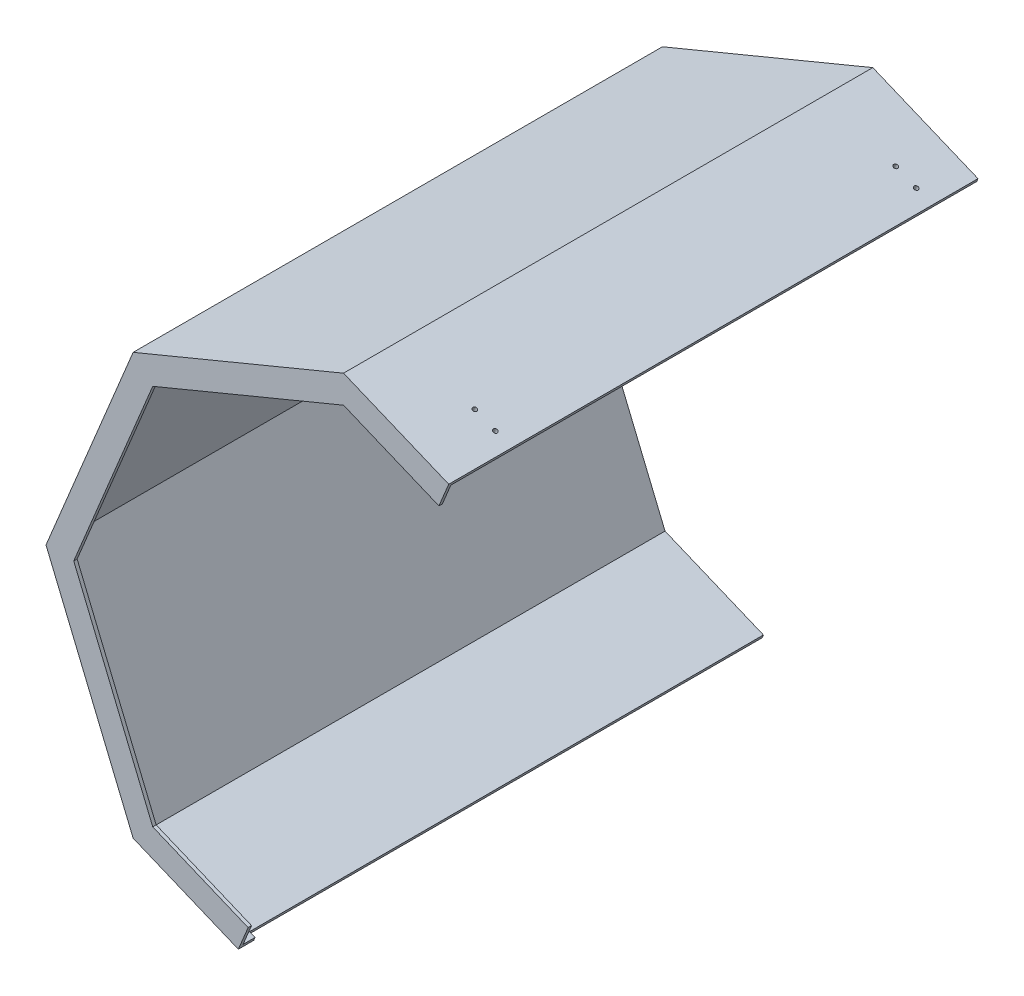
from build123d import *

# Parameters (mm, degrees)
BOSS_EXTRUDE1_DEPTH   = 310
SHELL1_T              = -2
CUT_EXTRUDE1_DEPTH    = 10
CUT_EXTRUDE2_DEPTH    = 397.026111511
SKETCH4_R             = 3
BOSS_EXTRUDE2_DEPTH   = 2
M3_TAPPED_HOLE1_D     = 2.5
M3_TAPPED_HOLE1_DEPTH = 4
CUT_EXTRUDE3_REACH    = 466.348
SKETCH7_W             = 3.5
SKETCH7_H             = 301


with BuildPart() as part:
    # Sketch1 → Boss-Extrude1 (new body)
    with BuildSketch(Plane.XY):
        Polygon((-174.265144247, 0), (-123.224065222, -123.224065222), (0, -174.265144247), (123.224065222, -123.224065222), (174.265144247, 0), (123.224065222, 123.224065222), (0, 174.265144247), (-123.224065222, 123.224065222), align=None)
    extrude(amount=BOSS_EXTRUDE1_DEPTH)

    # Shell1
    shell1_openings = [part.faces().sort_by_distance(p)[0] for p in [
        (0, 0, 0),
    ]]
    offset(amount=SHELL1_T, openings=shell1_openings, kind=Kind.INTERSECTION)

    # Sketch2 → Cut-Extrude1 (cut)
    with BuildSketch(Plane.XY.offset(310)):
        Polygon((111.743562251, 111.743562251), (0, 158.029261243), (-111.743562251, 111.743562251), (-158.029261243, 0), (-111.743562251, -111.743562251), (0, -158.029261243), (111.743562251, -111.743562251), (158.029261243, 0), align=None)
    extrude(amount=-CUT_EXTRUDE1_DEPTH, mode=Mode.SUBTRACT)

    # Sketch3 → Cut-Extrude2 (cut, through all)
    with BuildSketch(Plane.XY.offset(310)):
        Polygon((70.138181093, 169.328548035), (-63.801020235, -154.029288344), (130.028007017, -234.315900213), (263.967208344, 89.041936166), align=None)
    extrude(amount=-CUT_EXTRUDE2_DEPTH, mode=Mode.SUBTRACT)

    # Sketch4 → Boss-Extrude2 (add)
    with BuildSketch(Plane(origin=(60.846665746, 146.896845669, 0), x_dir=(0.9238795325112958, -0.38268343236506785, 0), z_dir=(-0.38268343236506785, -0.9238795325112958, 0))):
        with Locations((-23.217589358, 273.25)):
            Circle(SKETCH4_R)
        with Locations((-10.217589358, 273.25)):
            Circle(SKETCH4_R)
        with Locations((-10.217589358, 26.75)):
            Circle(SKETCH4_R)
        with Locations((-23.217589358, 26.75)):
            Circle(SKETCH4_R)
    extrude(amount=BOSS_EXTRUDE2_DEPTH)

    # M3 Tapped Hole1
    with Locations(Plane(origin=(61.612032611, 148.744604734, 0), x_dir=(0.9238795325112958, -0.38268343236506785, 0), z_dir=(0.38268343236506785, 0.9238795325112958, 0))):
        with Locations((-23.217589358, -26.75), (-10.217589358, -26.75), (-23.217589358, -273.25), (-10.217589358, -273.25)):
            Hole(M3_TAPPED_HOLE1_D / 2, depth=M3_TAPPED_HOLE1_DEPTH)

    # Sketch7 → Cut-Extrude3 (cut, up to next)
    with BuildSketch(Plane(origin=(-61.612032611, -148.744604734, 0), x_dir=(0.9238795325112957, -0.38268343236506797, 0), z_dir=(-0.38268343236506797, -0.9238795325112957, 0)), mode=Mode.PRIVATE) as cut_extrude3_sk1:
        with Locations((-1.75, 150.5)):
            Rectangle(SKETCH7_W, SKETCH7_H)
    cut_extrude3_tool1 = extrude(cut_extrude3_sk1.sketch, amount=-CUT_EXTRUDE3_REACH, mode=Mode.PRIVATE) & part.part
    add(cut_extrude3_tool1.solids().sort_by_distance((-63.228822, -148.074909, 150.5))[0], mode=Mode.SUBTRACT)


solid = part.part
